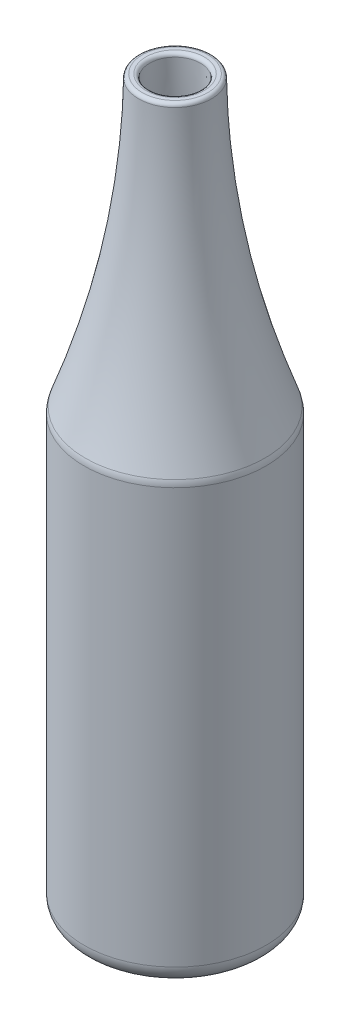
SolidWorks part; units mm, degrees
material "玻璃"
ref_plane "Front Plane" through (0, 0, 0) normal (0, 0, 1) x (1, 0, 0)
ref_plane "Top Plane" through (0, 0, 0) normal (0, 1, 0) x (1, 0, 0)
ref_plane "Right Plane" through (0, 0, 0) normal (1, 0, 0) x (0, 0, -1)
sketch "Sketch1" plane through (0, 0, 0) normal (0, 0, 1) x (1, 0, 0)
  line L0 (-93.0393, 135.7472) -> (-93.0393, -64.2528)
  line L1 (-118.0393, 55.7472) -> (-118.0393, -64.2528)
  line L2 (-118.0393, -64.2528) -> (-93.0393, -64.2528)
  line L3 (-103.0393, 135.7472) -> (-93.0393, 135.7472)
  spline S0 degree 2 poles (-118.0393, 55.7472) (-103.478, 95.0909) (-103.0393, 135.7472) knots 0 0 0 0.941503 0.941503 0.941503
  dimension "D1" = 120
  dimension "D2" = 10
  dimension "D3" = 200
  dimension "D4" = 25
revolve "Revolve1" add sketch "Sketch1" angle 360 about L0
shell "Shell1" thickness 3
fillet "Fillet1" radius 5 2 edges at (-93.0393, 55.7472, 25) (-93.0393, -64.2528, 25)
fillet "Fillet2" radius 1 2 edges at (-93.0393, 135.7472, 10) (-93.0393, 135.7472, 6.9998)
